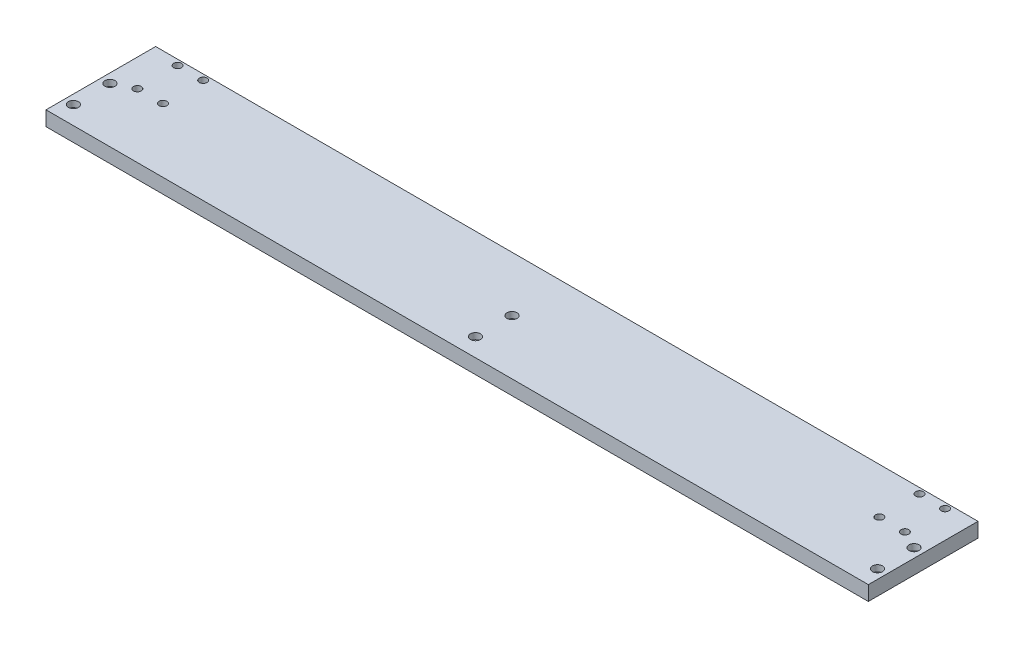
SolidWorks part; units mm, degrees
ref_plane "前视基准面" through (0, 0, 0) normal (0, 0, 1) x (1, 0, 0)
ref_plane "上视基准面" through (0, 0, 0) normal (0, 1, 0) x (1, 0, 0)
ref_plane "右视基准面" through (0, 0, 0) normal (1, 0, 0) x (0, 0, -1)
sketch "草图1" plane through (0, 0, 0) normal (0, 1, 0) x (1, 0, 0)
  line L1 (-450, 60) -> (450, 60)
  line L2 (-450, 60) -> (-450, -60)
  line L3 (-450, -60) -> (450, -60)
  line L4 (450, 60) -> (450, -60)
  line L5 (-450, 60) -> (450, -60) construction
  line L6 (-450, -60) -> (450, 60) construction
  point P0 (0, 0)
  dimension "D1" = 900
  dimension "D2" = 120
extrude "凸台-拉伸1" add sketch "草图1" along normal blind 16
hole_wizard "Ø8.5 (8.5) 直径孔1" positions "草图5" profile "草图6" hole size "Ø8.5" standard "GB" end condition through all
sketch "草图5" plane through (0, 16, 0) normal (0, 1, 0) x (1, 0, 0)
  line L0 (406, 138.7998) -> (406, 32) construction
  line L1 (406, 32) -> (212.9333, 32) construction
  line L2 (450, -60) -> (450, 60) construction
  line L3 (-450, -60) -> (450, -60) construction
  point P0 (392, 54)
  point P2 (420, 54)
  point P4 (392, 10)
  point P6 (420, 10)
  dimension "D1" = 28
  dimension "D2" = 44
  dimension "D3" = 30
  dimension "D4" = 70
sketch "草图6" plane through (392, 16, -54) normal (1, 0, 0) x (0, 0, 1)
  line L0 (0, 0) -> (0, 16)
  line L1 (0, 16) -> (4.25, 16)
  line L2 (4.25, 16) -> (4.25, 0)
  line L5 (4.25, 0) -> (0, 0)
  line L11 (0, -6.35) -> (0, 107.95) construction
  dimension "通孔孔直径" = 8.5
  dimension "通孔孔深度" = 16
hole_wizard "打孔尺寸(%根据)内六角圆柱头螺钉的类型1" positions "草图7" profile "草图8" counterbore size "M6" standard "GB" end condition through all
sketch "草图7" plane through (0, 16, 0) normal (0, 1, 0) x (1, 0, 0)
  line L0 (-450, -20) -> (-385.8695, -20) construction
  line L1 (-450, 60) -> (-450, -60) construction
  line L2 (450, 60) -> (-450, 60) construction
  point P0 (-440, 0)
  point P2 (-440, -40)
  dimension "D1" = 40
  dimension "D2" = 10
  dimension "D3" = 60
sketch "草图8" plane through (-440, 16, 0) normal (1, 0, 0) x (0, 0, 1)
  line L0 (0, 0) -> (0, 16)
  line L1 (0, 16) -> (3.3, 16)
  line L3 (3.3, 16) -> (3.3, 6.8)
  line L4 (3.3, 6.8) -> (5.5, 6.8)
  line L5 (5.5, 6.8) -> (5.5, 0)
  line L7 (5.5, 0) -> (0, 0)
  line L11 (0, -6.35) -> (0, 107.95) construction
  dimension "通孔孔直径" = 6.6
  dimension "通孔孔深度" = 16
  dimension "柱形沉头孔直径" = 11
  dimension "柱形沉头孔深度" = 6.8
pattern_linear "阵列(线性)1" count 3 spacing 440 along (1, 0, 0) of "打孔尺寸(%根据)内六角圆柱头螺钉的类型1"
mirror "镜向1" about plane through (0, 0, 0) normal (1, 0, 0) of "Ø8.5 (8.5) 直径孔1"
